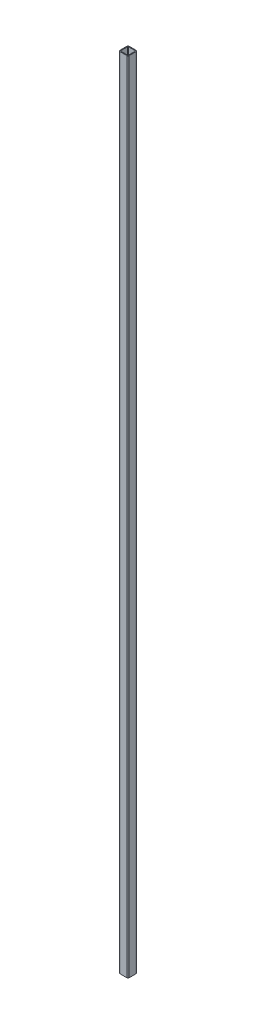
from build123d import *

# Parameters (mm, degrees)
COLD_FORMED_HOLLOW_STRUCTURAL_SQUARE_STE_DEPTH = 10370


with BuildPart() as part:
    # Sketch12 → Cold-formed Hollow Structural Square Steel(gb t6728-2002) 120×120×10(1) (new body)
    with BuildSketch(Plane(origin=(0, 0, 0), x_dir=(-1, 0, 0), z_dir=(0, 1, 0))):
        with BuildLine():
            Line((-44, -60), (44, -60))
            ThreePointArc((44, -60), (55.313708499, -55.313708499), (60, -44))
            Line((60, -44), (60, 44))
            ThreePointArc((60, 44), (55.313708499, 55.313708499), (44, 60))
            Line((44, 60), (-44, 60))
            ThreePointArc((-44, 60), (-55.313708499, 55.313708499), (-60, 44))
            Line((-60, 44), (-60, -44))
            ThreePointArc((-60, -44), (-55.313708499, -55.313708499), (-44, -60))
        make_face()
        with BuildLine():
            Line((-44, -50), (44, -50))
            ThreePointArc((44, -50), (48.242640687, -48.242640687), (50, -44))
            Line((50, -44), (50, 44))
            ThreePointArc((50, 44), (48.242640687, 48.242640687), (44, 50))
            Line((44, 50), (-44, 50))
            ThreePointArc((-44, 50), (-48.242640687, 48.242640687), (-50, 44))
            Line((-50, 44), (-50, -44))
            ThreePointArc((-50, -44), (-48.242640687, -48.242640687), (-44, -50))
        make_face(mode=Mode.SUBTRACT)
    extrude(amount=COLD_FORMED_HOLLOW_STRUCTURAL_SQUARE_STE_DEPTH)


solid = part.part
